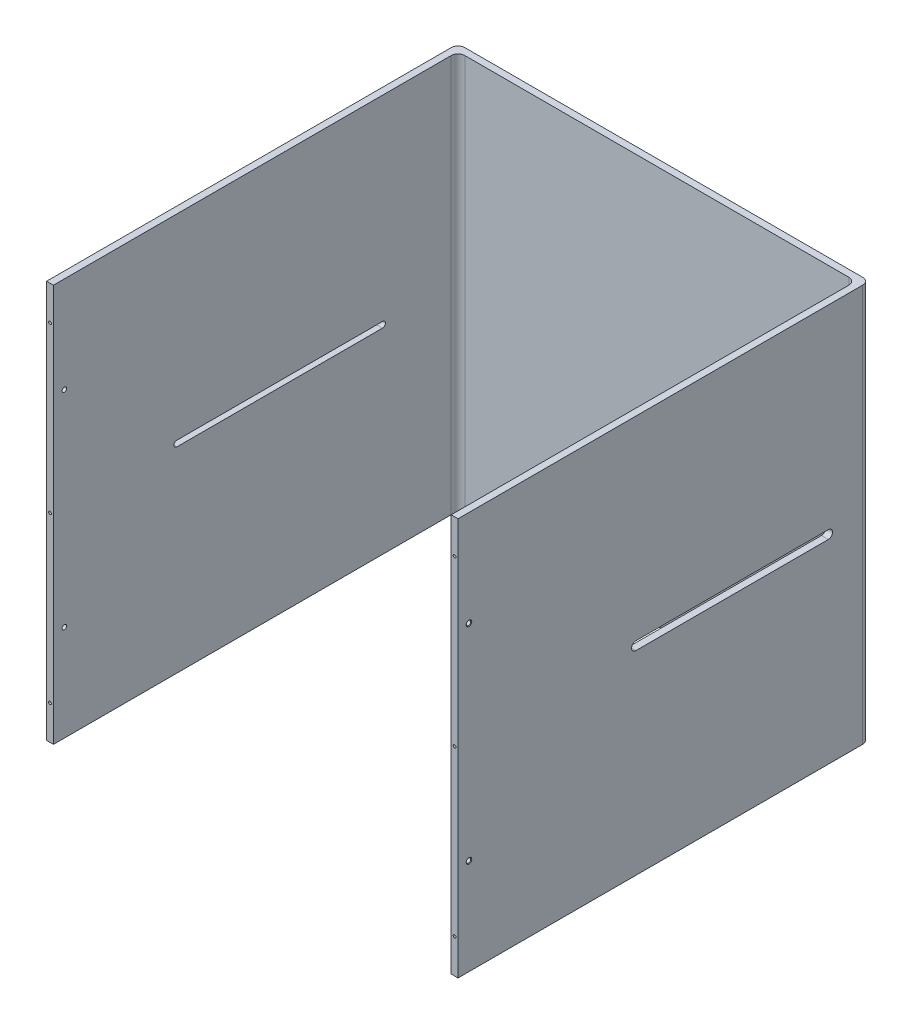
from build123d import *

# Parameters (mm, degrees)
BOSS_EXTRUDE1_DEPTH         = 290
M2_5_TAPPED_HOLE1_D         = 2.05
M2_5_TAPPED_HOLE1_DEPTH     = 7.25
M2_5_TAPPED_HOLE1_TIP       = 0.615882135
CUT_EXTRUDE2_DEPTH          = 41
CUT_EXTRUDE3_DEPTH          = 56
M4_TAPPED_HOLE1_D           = 3.3
M4_TAPPED_HOLE1_CSINK_D     = 4.05
M4_TAPPED_HOLE1_CSINK_ANGLE = 90
M2_5_TAPPED_HOLE2_D         = 2.05
M2_5_TAPPED_HOLE2_DEPTH     = 7.25
M2_5_TAPPED_HOLE2_TIP       = 0.615882135


with BuildPart() as part:
    # Sketch1 → Boss-Extrude1 (new body)
    with BuildSketch(Plane(origin=(0, 0, 0), x_dir=(1, 0, 0), z_dir=(0, 1, 0))):
        with BuildLine():
            Line((-138.105758434, 176.332217748), (151.894241566, 176.332217748))
            ThreePointArc((151.894241566, 176.332217748), (155.429775472, 174.867751654), (156.894241566, 171.332217748))
            Line((156.894241566, 171.332217748), (156.894241566, -123.667782252))
            Line((156.894241566, -123.667782252), (151.894241566, -123.667782252))
            Line((151.894241566, -123.667782252), (151.894241566, 166.332217748))
            ThreePointArc((151.894241566, 166.332217748), (150.429775472, 169.867751654), (146.894241566, 171.332217748))
            Line((146.894241566, 171.332217748), (-133.105758434, 171.332217748))
            ThreePointArc((-133.105758434, 171.332217748), (-136.64129234, 169.867751654), (-138.105758434, 166.332217748))
            Line((-138.105758434, 166.332217748), (-138.105758434, -123.667782252))
            Line((-138.105758434, -123.667782252), (-143.105758434, -123.667782252))
            Line((-143.105758434, -123.667782252), (-143.105758434, 171.332217748))
            ThreePointArc((-143.105758434, 171.332217748), (-141.64129234, 174.867751654), (-138.105758434, 176.332217748))
        make_face()
    extrude(amount=BOSS_EXTRUDE1_DEPTH)

    # M2.5 Tapped Hole1
    with Locations(Plane.XY.offset(123.667782252)):
        with Locations((-140.605758434, 145), (-140.605758434, 265), (-140.605758434, 25), (154.394241566, 145), (154.394241566, 265), (154.394241566, 25)):
            Hole(M2_5_TAPPED_HOLE1_D / 2, depth=M2_5_TAPPED_HOLE1_DEPTH)
            with Locations((0, 0, -(M2_5_TAPPED_HOLE1_DEPTH + M2_5_TAPPED_HOLE1_TIP / 2))):  # 118° drill point
                Cone(0, M2_5_TAPPED_HOLE1_D / 2, M2_5_TAPPED_HOLE1_TIP, mode=Mode.SUBTRACT)

    # Sketch5 → Cut-Extrude2 (cut)
    with BuildSketch(Plane.ZY.offset(143.105758434)):
        with BuildLine():
            Line((-116.332217748, 147.1), (33.667782252, 147.1))
            ThreePointArc((33.667782252, 147.1), (35.767782252, 145), (33.667782252, 142.9))
            Line((33.667782252, 142.9), (-116.332217748, 142.9))
            ThreePointArc((-116.332217748, 142.9), (-118.432217748, 145), (-116.332217748, 147.1))
        make_face()
    extrude(amount=-CUT_EXTRUDE2_DEPTH, mode=Mode.SUBTRACT)

    # Sketch6 → Cut-Extrude3 (cut)
    with BuildSketch(Plane(origin=(156.894241566, 0, 0), x_dir=(0, 0, -1), z_dir=(1, 0, 0))):
        with BuildLine():
            Line((6.018226887, 148.1), (146.332217748, 148.1))
            ThreePointArc((146.332217748, 148.1), (149.432217748, 145), (146.332217748, 141.9))
            Line((146.332217748, 141.9), (6.018226887, 141.9))
            ThreePointArc((6.018226887, 141.9), (2.918226887, 145), (6.018226887, 148.1))
        make_face()
    extrude(amount=-CUT_EXTRUDE3_DEPTH, mode=Mode.SUBTRACT)

    # M4 Tapped Hole1 (through all)
    with Locations(Plane(origin=(156.894241566, 0, 0), x_dir=(0, 0, -1), z_dir=(1, 0, 0))):
        with Locations((-115.667782252, 220), (-115.667782252, 70)):
            CounterSinkHole(M4_TAPPED_HOLE1_D / 2, M4_TAPPED_HOLE1_CSINK_D / 2, counter_sink_angle=M4_TAPPED_HOLE1_CSINK_ANGLE)

    # M2.5 Tapped Hole2
    with Locations(Plane(origin=(0, 0, 0), x_dir=(-1, 0, 0), z_dir=(0, -1, 0))):
        with Locations((-154.394241566, 136.332217748), (-154.394241566, 86.332217748), (-154.394241566, 6.332217748), (-154.394241566, -73.667782252), (-121.894241566, 173.832217748), (-51.894241566, 173.832217748), (38.105758434, 173.832217748), (108.105758434, 173.832217748), (140.605758434, -73.667782252), (140.605758434, 6.332217748), (140.605758434, 86.332217748), (140.605758434, 136.332217748)):
            Hole(M2_5_TAPPED_HOLE2_D / 2, depth=M2_5_TAPPED_HOLE2_DEPTH)
            with Locations((0, 0, -(M2_5_TAPPED_HOLE2_DEPTH + M2_5_TAPPED_HOLE2_TIP / 2))):  # 118° drill point
                Cone(0, M2_5_TAPPED_HOLE2_D / 2, M2_5_TAPPED_HOLE2_TIP, mode=Mode.SUBTRACT)


solid = part.part
